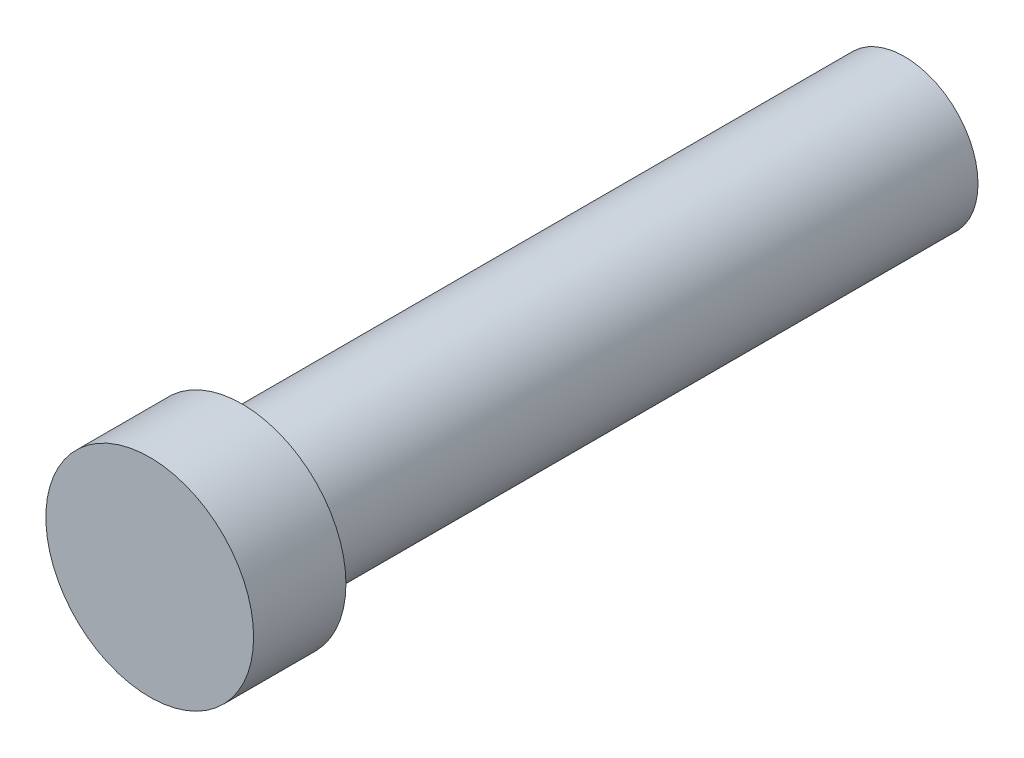
SolidWorks part; units mm, degrees
ref_plane "前视基准面" through (0, 0, 0) normal (0, 0, 1) x (1, 0, 0)
ref_plane "上视基准面" through (0, 0, 0) normal (0, 1, 0) x (1, 0, 0)
ref_plane "右视基准面" through (0, 0, 0) normal (1, 0, 0) x (0, 0, -1)
sketch "草图1" plane through (0, 0, 0) normal (0, 0, 1) x (1, 0, 0)
  circle A0 centre (0, 0) radius 1.59
  dimension "D1" = 3.18
extrude "凸台-拉伸1" add sketch "草图1" along normal blind 14.35
sketch "草图2" plane through (0, 0, 14.35) normal (0, 0, 1) x (1, 0, 0)
  circle A2 centre (0, 0) radius 2.25
extrude "凸台-拉伸2" add sketch "草图2" along normal blind 2 separate body
sketch "草图3" plane through (0, 0, 16.35) normal (0, 0, 1) x (1, 0, 0)
  circle A0 centre (0, 0) radius 2.25
